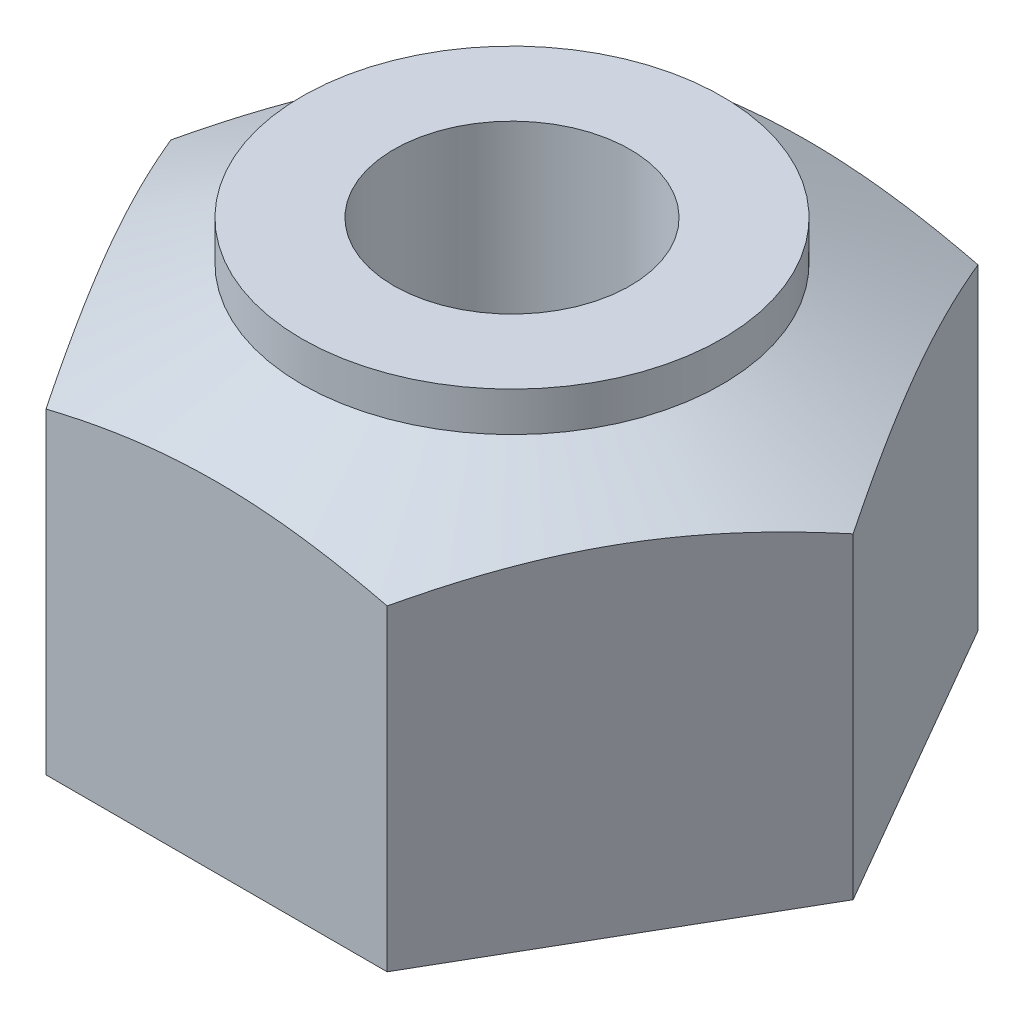
from build123d import *

# Parameters (mm, degrees)
BOSS_EXTRUDE1_DEPTH    = 24
SKETCH_2_2_R           = 16
BOSS_EXTRUDE2_DEPTH    = 8
SKETCH_3_3_R           = 17.5
SKETCH_3_3_R_2         = 9
SKETCH_3_3_R_3         = 6
CUT_EXTRUDE1_DEPTH     = 14
BOSS_EXTRUDE3_DEPTH    = 5
SKETCH_3_4_R           = 6
CUT_EXTRUDE3_DEPTH     = 47.960089438
CUT_EXTRUDE2_START     = -32
SKETCH_3_3_2_R         = 9
CUT_EXTRUDE2_DEPTH     = 15
CUT_EXTRUDE4_START     = 5
SKETCH_2_2_2_OUTSIDE_W = 89.63
SKETCH_2_2_2_OUTSIDE_H = 82.668
SKETCH_2_2_2_OUTSIDE_R = 16
CUT_EXTRUDE4_DEPTH     = 5
CUT_EXTRUDE4_DRAFT     = -64


with BuildPart() as part:
    # Sketch 1_2 → Boss-Extrude1 (new body)
    with BuildSketch(Plane.XZ):
        Polygon((-12.990381057, 22.5), (12.990381057, 22.5), (25.980762114, 0), (12.990381057, -22.5), (-12.990381057, -22.5), (-25.980762114, 0), align=None)
    extrude(amount=BOSS_EXTRUDE1_DEPTH)

    # Sketch 2_2 → Boss-Extrude2 (add)
    with BuildSketch(Plane(origin=(0, 0, 0), x_dir=(-1, 0, 0), z_dir=(0, 1, 0))):
        with Locations(Location((0, 0, 0), (0, 0, 90))):
            Circle(SKETCH_2_2_R)
    extrude(amount=BOSS_EXTRUDE2_DEPTH)

    # Sketch 3_3 → Cut-Extrude1 (cut)
    # profile 1 of 2: a face of its own
    with BuildSketch(Plane(origin=(0, -24, 0), x_dir=(-1, 0, 0), z_dir=(0, -1, 0))):
        with Locations(Location((0, 0, 0), (0, 0, 90))):
            Circle(SKETCH_3_3_R)
        Circle(SKETCH_3_3_R_2, mode=Mode.SUBTRACT)
    # profile 2 of 2: a face of its own
    with BuildSketch(Plane(origin=(0, -24, 0), x_dir=(-1, 0, 0), z_dir=(0, -1, 0))):
        Circle(SKETCH_3_3_R_2)
        with Locations(Location((0, 0, 0), (0, 0, 90))):
            Circle(SKETCH_3_3_R_3, mode=Mode.SUBTRACT)
    extrude(amount=-CUT_EXTRUDE1_DEPTH, mode=Mode.SUBTRACT)

    # Sketch 1_2 2 → Boss-Extrude3 (add)
    with BuildSketch(Plane.XZ):
        Polygon((-12.990381057, 22.5), (12.990381057, 22.5), (25.980762114, 0), (12.990381057, -22.5), (-12.990381057, -22.5), (-25.980762114, 0), align=None)
    extrude(amount=-BOSS_EXTRUDE3_DEPTH)

    # 草图3<4> → Cut-Extrude3 (cut, through all)
    with BuildSketch(Plane(origin=(0, -24, 0), x_dir=(-1, 0, 0), z_dir=(0, -1, 0))):
        with Locations(Location((0, 0, 0), (0, 0, 90))):
            Circle(SKETCH_3_4_R)
    extrude(amount=-CUT_EXTRUDE3_DEPTH, mode=Mode.SUBTRACT)

    # Sketch 3_3 2 → Cut-Extrude2 (cut)
    with BuildSketch(Plane(origin=(0, -24, 0), x_dir=(-1, 0, 0), z_dir=(0, -1, 0)).offset(CUT_EXTRUDE2_START)):
        with Locations(Location((0, 0, 0), (0, 0, 270))):
            Circle(SKETCH_3_3_2_R)
    extrude(amount=CUT_EXTRUDE2_DEPTH, mode=Mode.SUBTRACT)


with BuildPart() as cut_extrude4_tool:
    # Sketch 2_2 2 outside → Cut-Extrude4 (with draft: the straight prism first)
    with BuildSketch(Plane(origin=(0, 0, 0), x_dir=(-1, 0, 0), z_dir=(0, 1, 0)).offset(CUT_EXTRUDE4_START)):
        Rectangle(SKETCH_2_2_2_OUTSIDE_W, SKETCH_2_2_2_OUTSIDE_H)
        with Locations(Location((0, 0, 0), (0, 0, 90))):
            Circle(SKETCH_2_2_2_OUTSIDE_R, mode=Mode.SUBTRACT)
    extrude(amount=-CUT_EXTRUDE4_DEPTH)
    # Cut-Extrude4: the draft: its side faces are tilted about the plane it starts from
    cut_extrude4_sides = [cut_extrude4_tool.faces().sort_by_distance(p)[0] for p in [
        (0, 2.5, -41.334),
        (-44.815, 2.5, 0),
        (0, 2.5, 41.334),
        (44.815, 2.5, 0),
        (0, 2.5, -16),
    ]]
    draft(cut_extrude4_sides, Plane(origin=(0, 0, 0), x_dir=(-1, 0, 0), z_dir=(0, 1, 0)).offset(CUT_EXTRUDE4_START), CUT_EXTRUDE4_DRAFT)


with BuildPart() as part_1:
    add(part.part)

    # Cut-Extrude4: cut by cut_extrude4_tool
    add(cut_extrude4_tool.part, mode=Mode.SUBTRACT)


solid = part_1.part
